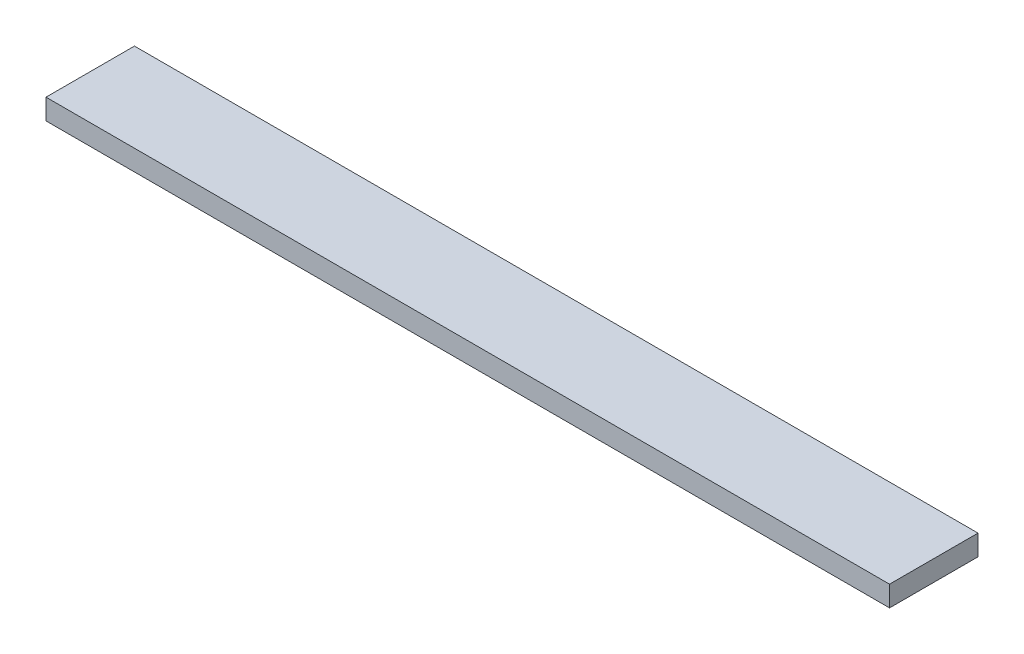
SolidWorks part; units mm, degrees
material "塑料"
ref_plane "Front Plane" through (0, 0, 0) normal (0, 0, 1) x (1, 0, 0)
ref_plane "Top Plane" through (0, 0, 0) normal (0, 1, 0) x (1, 0, 0)
ref_plane "Right Plane" through (0, 0, 0) normal (1, 0, 0) x (0, 0, -1)
sketch "Sketch1" plane through (0, 0, 0) normal (0, 1, 0) x (1, 0, 0)
  line L1 (0, 2.15) -> (41, 2.15)
  line L2 (0, 2.15) -> (0, -2.15)
  line L3 (0, -2.15) -> (41, -2.15)
  line L4 (41, 2.15) -> (41, -2.15)
  point P4 (0, 0)
  dimension "D1" = 41
  dimension "D2" = 4.3
extrude "Boss-Extrude1" add sketch "Sketch1" along normal blind 1
